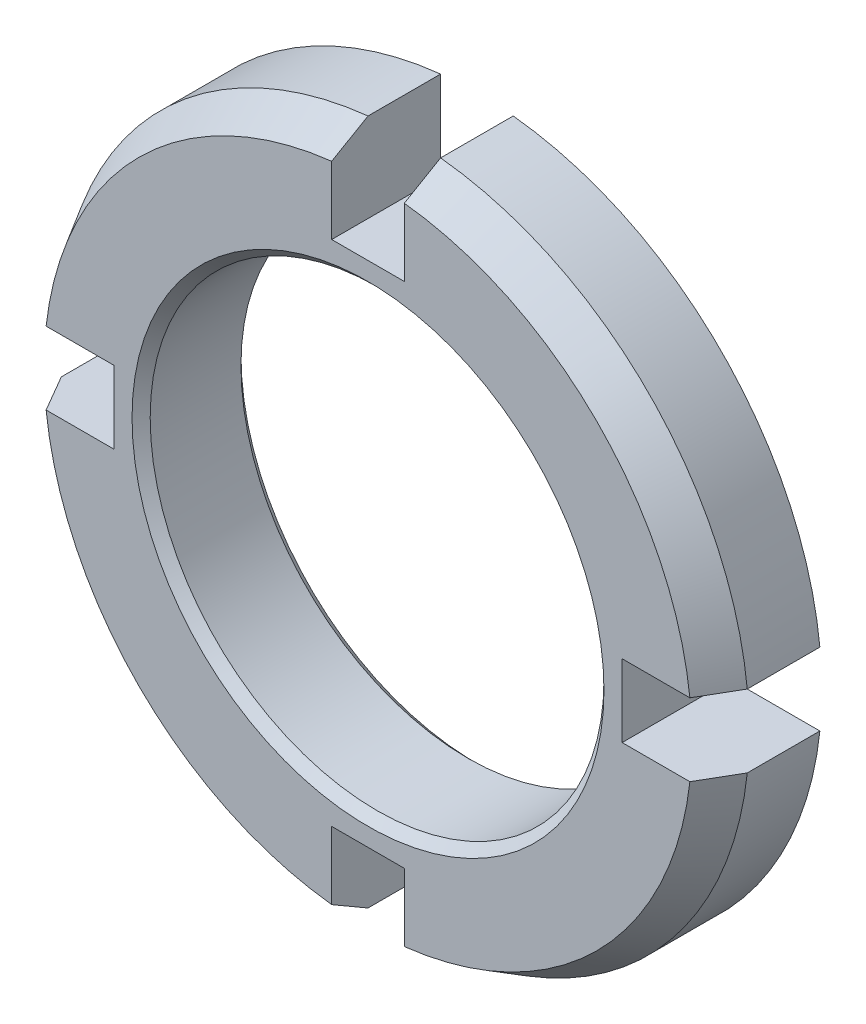
from build123d import *
from OCP.BRepFilletAPI import BRepFilletAPI_MakeChamfer

# Parameters (mm, degrees)
SKETCH1_R           = 19
SKETCH1_R_2         = 12.5
BOSS_EXTRUDE1_DEPTH = 6
SKETCH2_W           = 6
SKETCH2_H           = 4
CUT_EXTRUDE1_DEPTH  = 6
CIRPATTERN1_COUNT   = 4
CHAMFER1_SIZE       = 0.5
CHAMFER2_SIZE       = 2
CHAMFER2_SIZE2      = 1.154700538


with BuildPart() as part:
    # Sketch1 → Boss-Extrude1 (new body)
    with BuildSketch(Plane.XY):
        Circle(SKETCH1_R)
        Circle(SKETCH1_R_2, mode=Mode.SUBTRACT)
    extrude(amount=BOSS_EXTRUDE1_DEPTH)

    # Sketch2 → Cut-Extrude1 (cut)
    with BuildSketch(Plane(origin=(14, 0, 0), x_dir=(0, 0, -1), z_dir=(1, 0, 0))):
        with Locations((-3, 0)):
            Rectangle(SKETCH2_W, SKETCH2_H)
    cut_extrude1 = extrude(amount=CUT_EXTRUDE1_DEPTH, mode=Mode.SUBTRACT)

    # CirPattern1: Cut-Extrude1 ×4 about axis
    cirpattern1_axis = Axis((0, 0, 0), (0, 0, 1))
    for i in range(1, CIRPATTERN1_COUNT):
        add(cut_extrude1.rotate(cirpattern1_axis, i * 360 / CIRPATTERN1_COUNT), mode=Mode.SUBTRACT)

    # Chamfer1
    chamfer1_edges = [part.edges().sort_by_distance(p)[0] for p in [
        (-12.5, 0, 0),
        (-12.5, 0, 6),
    ]]
    chamfer(chamfer1_edges, length=CHAMFER1_SIZE)

    # Chamfer2: one chamfer whose edges measure the first distance from different faces: ONE call of the kernel's chamfer builder (chamfer() names one face for all edges)
    chamfer2_edges_1 = [part.edges().sort_by_distance(p)[0] for p in [
        (13.435028843, -13.435028843, 6),
    ]]
    chamfer2_side_1 = [part.faces().sort_by_distance(p)[0] for p in [
        (13.435028843, -13.435028843, 3),
    ]]
    chamfer2_edges_2 = [part.edges().sort_by_distance(p)[0] for p in [
        (13.435028843, 13.435028843, 6),
    ]]
    chamfer2_side_2 = [part.faces().sort_by_distance(p)[0] for p in [
        (13.435028843, 13.435028843, 3),
    ]]
    chamfer2_edges_3 = [part.edges().sort_by_distance(p)[0] for p in [
        (-13.435028843, -13.435028843, 6),
    ]]
    chamfer2_side_3 = [part.faces().sort_by_distance(p)[0] for p in [
        (-13.435028843, -13.435028843, 3),
    ]]
    chamfer2_edges_4 = [part.edges().sort_by_distance(p)[0] for p in [
        (-13.435028843, 13.435028843, 6),
    ]]
    chamfer2_side_4 = [part.faces().sort_by_distance(p)[0] for p in [
        (-13.435028843, 13.435028843, 3),
    ]]
    chamfer2 = BRepFilletAPI_MakeChamfer(part.part.solid().wrapped)
    for e in chamfer2_edges_1:
        chamfer2.Add(CHAMFER2_SIZE, CHAMFER2_SIZE2, e.wrapped, chamfer2_side_1[0].wrapped)  # the first distance lies on this face
    for e in chamfer2_edges_2:
        chamfer2.Add(CHAMFER2_SIZE, CHAMFER2_SIZE2, e.wrapped, chamfer2_side_2[0].wrapped)  # the first distance lies on this face
    for e in chamfer2_edges_3:
        chamfer2.Add(CHAMFER2_SIZE, CHAMFER2_SIZE2, e.wrapped, chamfer2_side_3[0].wrapped)  # the first distance lies on this face
    for e in chamfer2_edges_4:
        chamfer2.Add(CHAMFER2_SIZE, CHAMFER2_SIZE2, e.wrapped, chamfer2_side_4[0].wrapped)  # the first distance lies on this face
    add(Compound.cast(chamfer2.Shape()), mode=Mode.REPLACE)


solid = part.part
